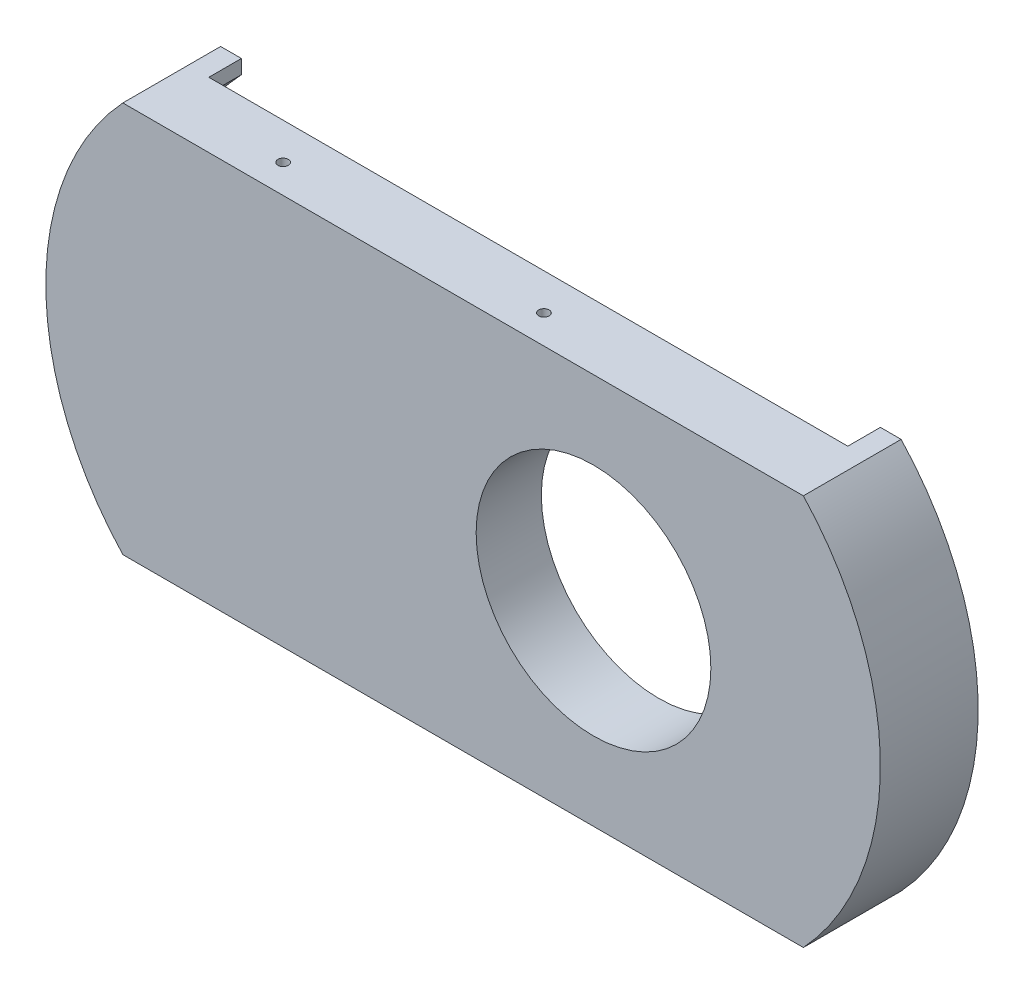
SolidWorks part; units mm, degrees
ref_plane "Front Plane" through (0, 0, 0) normal (0, 0, 1) x (1, 0, 0)
ref_plane "Top Plane" through (0, 0, 0) normal (0, 1, 0) x (1, 0, 0)
ref_plane "Right Plane" through (0, 0, 0) normal (1, 0, 0) x (0, 0, -1)
sketch "Sketch1" plane through (0, 0, 0) normal (0, 0, 1) x (1, 0, 0)
  line L0 (-10, 0) -> (10, 0) construction
  line L1 (-26.0935, 15) -> (26.0935, 15)
  line L2 (-26.0935, -15) -> (26.0935, -15)
  circle A0 centre (-10, 0) radius 2
  circle A1 centre (10, 0) radius 2
  arc A2 (-26.0935, 15) -> (-26.0935, -15) centre (-10, 0) ccw
  arc A5 (26.0935, -15) -> (26.0935, 15) centre (10, 0) ccw
  point P4 (0, 0)
  dimension "D2" = 4
  dimension "D3" = 44
  dimension "D4" = 15
  dimension "D1" = 20
  dimension "D5" = 10
extrude "Boss-Extrude1" add sketch "Sketch1" along normal blind 5
sketch "Sketch2" plane through (0, 0, 0) normal (0, 0, -1) x (-1, 0, 0)
  circle A0 centre (10, 0) radius 8.5
  dimension "D1" = 17
extrude "Cut-Extrude1" cut sketch "Sketch2" against normal blind 2
sketch "Sketch3" plane through (0, 0, 0) normal (0, 0, -1) x (-1, 0, 0)
  circle A0 centre (-10, 0) radius 9
  dimension "D1" = 18
extrude "Cut-Extrude2" cut sketch "Sketch3" against normal up to next
sketch "Sketch4" plane through (0, 0, 0) normal (0, 0, -1) x (-1, 0, 0)
  line L0 (0, 0) -> (0, 15) construction
  line L1 (26.0935, 15) -> (23.3795, 15)
  line L2 (-26.0935, -15) -> (-23.3795, -15)
  line L6 (26.0935, -15) -> (23.3795, -15)
  line L8 (-26.0935, 15) -> (-23.3795, 15)
  arc A0 (26.0935, -15) -> (26.0935, 15) centre (10, 0) ccw construction
  arc A2 (26.0935, -15) -> (26.0935, 15) centre (10, 0) ccw
  arc A6 (23.3795, 15) -> (23.3795, -15) centre (10, 0) cw
  arc A7 (26.0935, 15) -> (26.0935, -15) centre (10, 0) cw
  arc A8 (-26.0935, 15) -> (-26.0935, -15) centre (-10, 0) ccw
  arc A10 (-23.3795, 15) -> (-23.3795, -15) centre (-10, 0) ccw
  arc A11 (-26.0935, -15) -> (-26.0935, 15) centre (-10, 0) cw
  dimension "D1" = 20.1
  dimension "D2" = 10
extrude "Boss-Extrude2" add sketch "Sketch4" along normal blind 2.5
sketch "Sketch5" plane through (0, 0, 0) normal (0, 0, -1) x (-1, 0, 0)
  line L1 (-24.5, 18.2225) -> (24.5, 18.2225)
  line L2 (-24.5, 18.2225) -> (-24.5, -18.2225)
  line L3 (-24.5, -18.2225) -> (24.5, -18.2225)
  line L4 (24.5, 18.2225) -> (24.5, -18.2225)
  line L5 (-24.5, 18.2225) -> (24.5, -18.2225) construction
  line L6 (-24.5, -18.2225) -> (24.5, 18.2225) construction
  point P0 (0, 0)
  dimension "D1" = 49
extrude "Cut-Extrude3" cut sketch "Sketch5" along normal blind 11.5
sketch "Sketch6" plane through (0, 0, 0) normal (0, 0, 1) x (1, 0, 0)
  line L1 (10, 0) -> (21, 0) construction
  line L2 (10, 0) -> (10, 12.5) construction
  line L3 (10, 12.5) -> (21, 12.5) construction
  line L4 (21, 0) -> (21, 12.5) construction
  line L5 (-10, 0) -> (1, 0) construction
  line L6 (-10, 0) -> (-10, 12.5) construction
  line L7 (-10, 12.5) -> (1, 12.5) construction
  line L8 (1, 0) -> (1, 12.5) construction
  circle A0 centre (1, 12.5) radius 1.65
  circle A1 centre (21, 12.5) radius 1.65
  dimension "D4" = 3.3
  dimension "D1" = 12.5
  dimension "D2" = 11
  dimension "D3" = 12.5
hole_wizard "Ø0.8 (0.8) Diameter Hole1" positions "3DSketch1" profile "Sketch7" hole size "Ø0.8" standard "GB"
sketch3d "3DSketch1"
  point P0 (1, 12.5, 0)
  point P3 (21, 12.5, 0)
sketch "Sketch7" plane through (1, 12.5, 0) normal (1, 0, 0) x (0, 1, 0)
  line L0 (0, 0) -> (0, 1.2403)
  line L1 (0, 1.2403) -> (0.4, 1)
  line L2 (0.4, 1) -> (0.4, 0)
  line L5 (0.4, 0) -> (0, 0)
  line L10 (0, 1.2403) -> (-0.4, 1) construction
  line L11 (0, -6.35) -> (0, 107.95) construction
  dimension "孔直径" = 0.8
  dimension "孔深度" = 1
  dimension "导头角度" = 118
sketch "Sketch8" plane through (0, 0, 2) normal (0, 0, -1) x (-1, 0, 0)
  circle A0 centre (10, 0) radius 2
extrude "Boss-Extrude3" add sketch "Sketch8" against normal up to surface (3 mm away) up to face at (19, 0, 5)
sketch "Sketch9" plane through (0, 15, 0) normal (0, 1, 0) x (1, 0, 0)
  line L0 (10, -2.8) -> (4, -2.8) construction
  line L1 (-1.5, -2) -> (-18.5, -2) construction
  line L3 (1, 0) -> (19, 0) construction
  line L4 (-10, -2) -> (-10, -5) construction
  line L5 (26.0935, -5) -> (-26.0935, -5) construction
  line L6 (10, -2.8) -> (10, -5) construction
  line L7 (-10, -2.8) -> (-16, -2.8) construction
  circle A0 centre (-16, -2.8) radius 0.4
  circle A1 centre (4, -2.8) radius 0.4
  dimension "D2" = 0.8
  dimension "D1" = 6
  dimension "D3" = 2.2
hole_wizard "Ø0.8 (0.8) Diameter Hole2" positions "3DSketch2" profile "Sketch10" hole size "Ø0.8" standard "GB"
sketch3d "3DSketch2"
  point P0 (-16, 15, 2.8)
  point P3 (4, 15, 2.8)
sketch "Sketch10" plane through (-16, 15, 2.8) normal (1, 0, 0) x (0, 0, 1)
  line L0 (0, 0) -> (0, 1.2403)
  line L1 (0, 1.2403) -> (0.4, 1)
  line L2 (0.4, 1) -> (0.4, 0)
  line L5 (0.4, 0) -> (0, 0)
  line L10 (0, 1.2403) -> (-0.4, 1) construction
  line L11 (0, -6.35) -> (0, 107.95) construction
  dimension "孔直径" = 0.8
  dimension "孔深度" = 1
  dimension "导头角度" = 118
